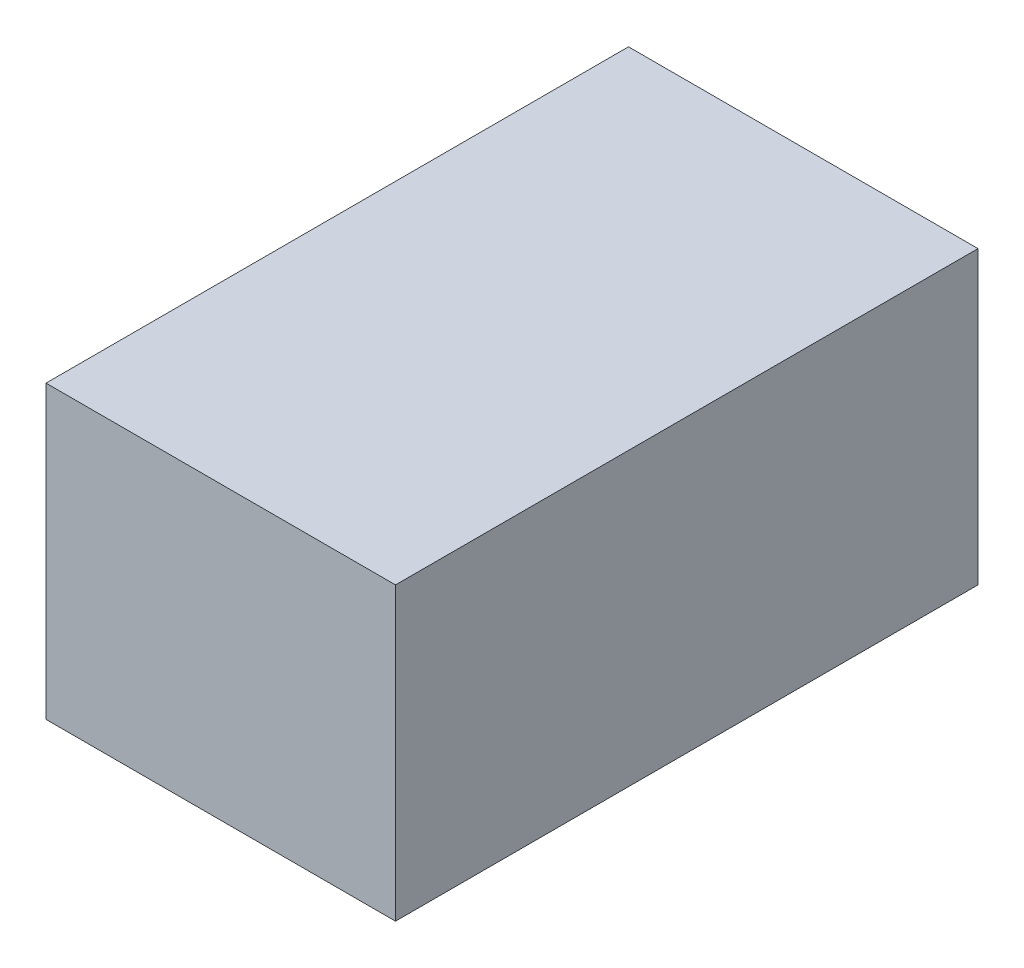
SolidWorks part; units mm, degrees
ref_plane "Front Plane" through (0, 0, 0) normal (0, 0, 1) x (1, 0, 0)
ref_plane "Top Plane" through (0, 0, 0) normal (0, 1, 0) x (1, 0, 0)
ref_plane "Right Plane" through (0, 0, 0) normal (1, 0, 0) x (0, 0, -1)
sketch "Sketch1" plane through (0, 0, 0) normal (0, 1, 0) x (1, 0, 0)
  line L1 (-30, 50) -> (30, 50)
  line L2 (-30, 50) -> (-30, -50)
  line L3 (-30, -50) -> (30, -50)
  line L4 (30, 50) -> (30, -50)
  line L5 (-30, 50) -> (30, -50) construction
  line L6 (-30, -50) -> (30, 50) construction
  point P0 (0, 0)
  dimension "D1" = 60
  dimension "D2" = 100
extrude "Boss-Extrude1" add sketch "Sketch1" along normal blind 50
